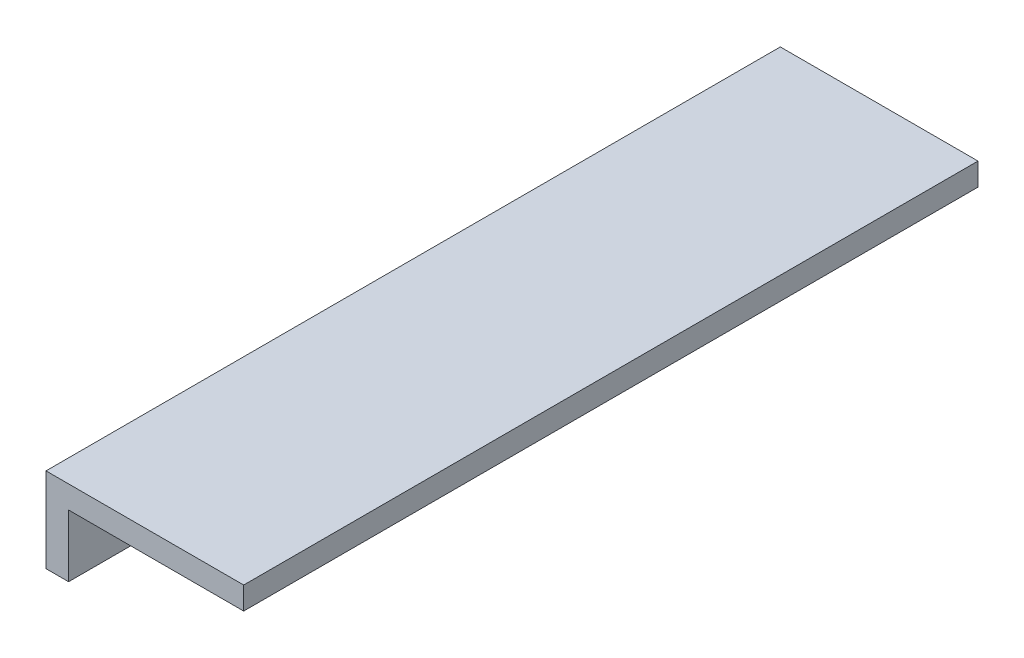
from build123d import *

# Parameters (mm, degrees)
EXTRUDE_1_DEPTH     = 260
SKETCH_2_W          = 50
SKETCH_2_H          = 15
CUT_EXTRUDE_1_DEPTH = 10


with BuildPart() as part:
    # 草图1 → 凸台-拉伸1 (new body)
    with BuildSketch(Plane.XY):
        Polygon((0, 0), (70, 0), (70, -8), (8, -8), (8, -30), (0, -30), align=None)
    extrude(amount=EXTRUDE_1_DEPTH)

    # 草图2 → 切除-拉伸1 (cut)
    with BuildSketch(Plane.ZY):
        with Locations((185, -22.5)):
            Rectangle(SKETCH_2_W, SKETCH_2_H)
    extrude(amount=-CUT_EXTRUDE_1_DEPTH, mode=Mode.SUBTRACT)


solid = part.part
